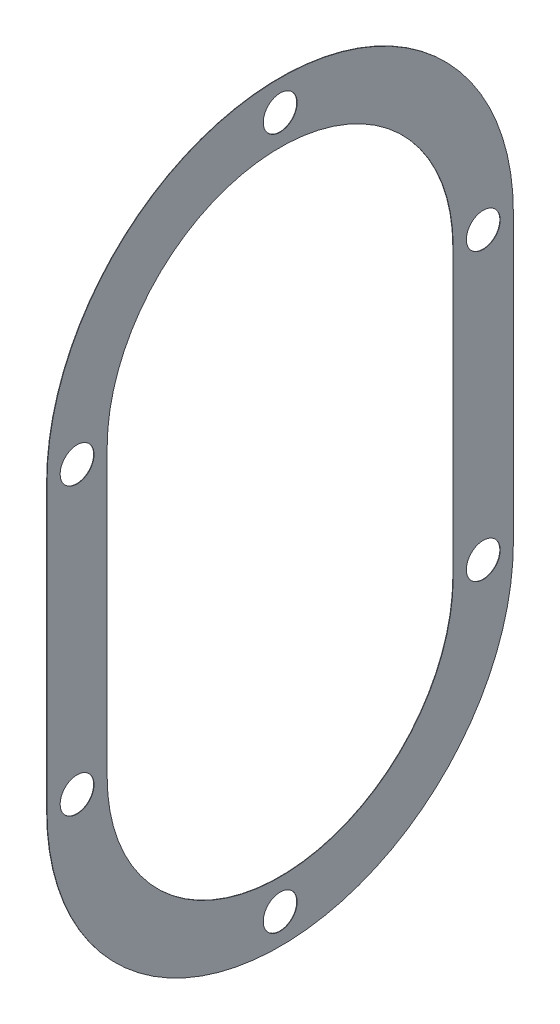
from build123d import *

# Parameters (mm, degrees)
SKETCH1_R           = 2.25
BOSS_EXTRUDE1_DEPTH = 0.05


with BuildPart() as part:
    # Sketch1 → Boss-Extrude1 (new body)
    with BuildSketch(Plane(origin=(0.05, 0, 0), x_dir=(0, 0, -1), z_dir=(1, 0, 0))):
        with BuildLine():
            Line((31, -19), (31, 19))
            ThreePointArc((31, 19), (0, 50), (-31, 19))
            Line((-31, 19), (-31, -19))
            ThreePointArc((-31, -19), (0, -50), (31, -19))
        make_face()
        with Locations(Location((27, -19, 0), (0, 0, 180))):
            Circle(SKETCH1_R, mode=Mode.SUBTRACT)
        with Locations(Location((27, 19, 0), (0, 0, 180))):
            Circle(SKETCH1_R, mode=Mode.SUBTRACT)
        with Locations(Location((0, 46, 0), (0, 0, 180))):
            Circle(SKETCH1_R, mode=Mode.SUBTRACT)
        with Locations(Location((-27, 19, 0), (0, 0, 180))):
            Circle(SKETCH1_R, mode=Mode.SUBTRACT)
        with Locations(Location((-27, -19, 0), (0, 0, 180))):
            Circle(SKETCH1_R, mode=Mode.SUBTRACT)
        with Locations(Location((0, -46, 0), (0, 0, 180))):
            Circle(SKETCH1_R, mode=Mode.SUBTRACT)
        with BuildLine():
            Line((23, 19), (23, -19))
            ThreePointArc((23, -19), (0, -42), (-23, -19))
            Line((-23, -19), (-23, 19))
            ThreePointArc((-23, 19), (0, 42), (23, 19))
        make_face(mode=Mode.SUBTRACT)
    extrude(amount=-BOSS_EXTRUDE1_DEPTH)


solid = part.part
